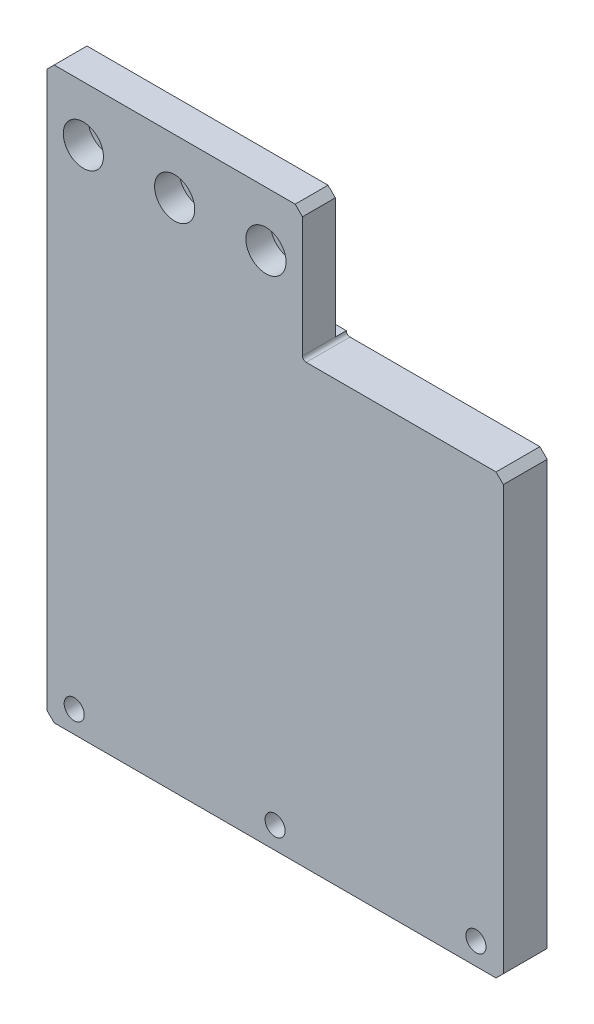
from build123d import *

# Parameters (mm, degrees)
SKETCH_1_W                = 125
SKETCH_1_H                = 156
EXTRUDE_1_DEPTH           = 12
SKETCH_2_W                = 55
SKETCH_2_H                = 36
CUT_EXTRUDE_1_DEPTH       = 101.669012114
SKETCH_3_W                = 70
SKETCH_3_H                = 35
CUT_EXTRUDE_2_DEPTH       = 3
HOLE_WIZARD_1_D           = 5.5
HOLE_WIZARD_1_CBORE_D     = 10
HOLE_WIZARD_1_CBORE_DEPTH = 5.7
HOLE_WIZARD_2_D           = 6.6
HOLE_WIZARD_2_CBORE_D     = 11
HOLE_WIZARD_2_CBORE_DEPTH = 6.8
CHAMFER_1_SIZE            = 2
FILLET_1_R                = 1


with BuildPart() as part:
    # 草图1 → 凸台-拉伸1 (new body)
    with BuildSketch(Plane.XY):
        Rectangle(SKETCH_1_W, SKETCH_1_H)
    extrude(amount=EXTRUDE_1_DEPTH)

    # 草图2 → 切除-拉伸1 (cut, through all)
    with BuildSketch(Plane.XY.offset(12)):
        with Locations((35, 60)):
            Rectangle(SKETCH_2_W, SKETCH_2_H)
    extrude(amount=-CUT_EXTRUDE_1_DEPTH, mode=Mode.SUBTRACT)

    # 草图3 → 切除-拉伸2 (cut)
    with BuildSketch(Plane(origin=(0, 0, 0), x_dir=(-1, 0, 0), z_dir=(0, 0, -1))):
        with Locations((27.5, 60.5)):
            Rectangle(SKETCH_3_W, SKETCH_3_H)
    extrude(amount=-CUT_EXTRUDE_2_DEPTH, mode=Mode.SUBTRACT)

    # 打孔尺寸(%根据)内六角圆柱头螺钉的类型1 (through all)
    with Locations(Plane(origin=(0, 0, 0), x_dir=(-1, 0, 0), z_dir=(0, 0, -1))):
        with Locations((-55, -72), (0, -72), (55, -72)):
            CounterBoreHole(HOLE_WIZARD_1_D / 2, HOLE_WIZARD_1_CBORE_D / 2, HOLE_WIZARD_1_CBORE_DEPTH)

    # 打孔尺寸(%根据)内六角圆柱头螺钉的类型2 (through all)
    with Locations(Plane(origin=(0, 0, 12), x_dir=(-1, 0, 0), z_dir=(0, 0, 1))):
        with Locations((2.5, -63), (27.5, -63), (52.5, -63)):
            CounterBoreHole(HOLE_WIZARD_2_D / 2, HOLE_WIZARD_2_CBORE_D / 2, HOLE_WIZARD_2_CBORE_DEPTH)

    # 倒角1
    chamfer_1_edges = [part.edges().sort_by_distance(p)[0] for p in [
        (62.5, 42, 6),
        (7.5, 78, 7.5),
        (62.5, -78, 6),
        (-62.5, -78, 6),
        (-62.5, 78, 7.5),
    ]]
    chamfer(chamfer_1_edges, length=CHAMFER_1_SIZE)

    # 圆角1
    fillet_1_edges = [part.edges().sort_by_distance(p)[0] for p in [
        (7.5, 42, 6),
    ]]
    fillet(fillet_1_edges, radius=FILLET_1_R)


solid = part.part
